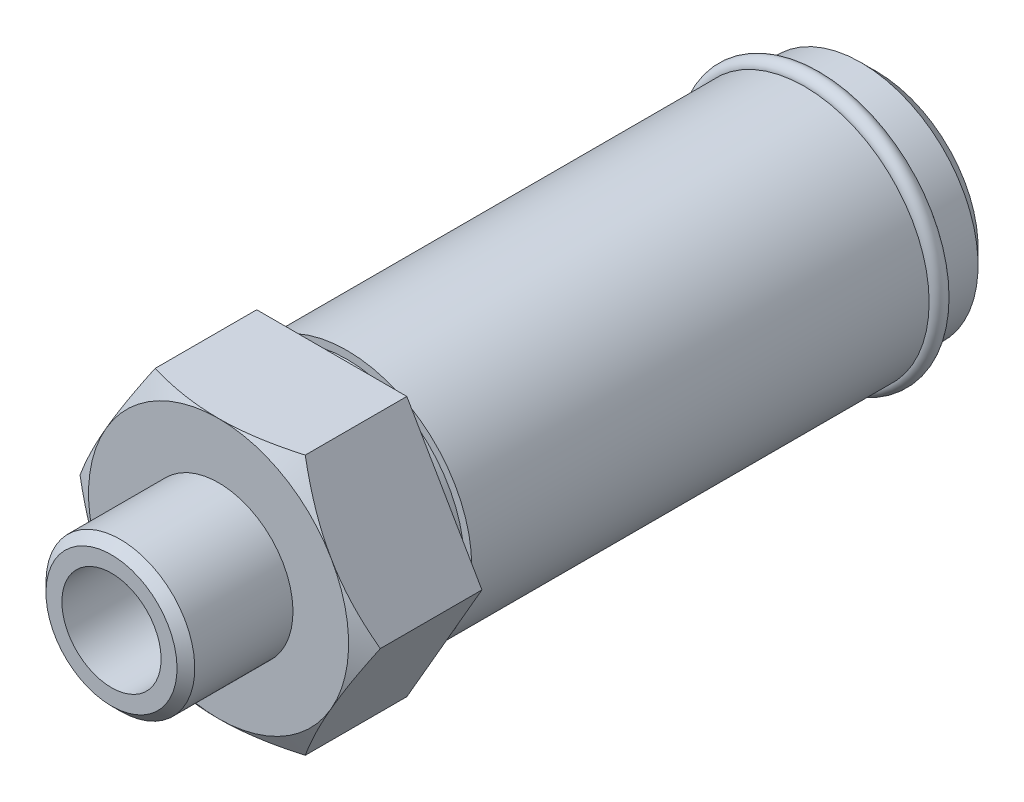
from build123d import *

# Parameters (mm, degrees)
CUT_EXTRUDE_START   = -7.4
SKETCH_2_R          = 17
CUT_EXTRUDE_1_DEPTH = 7.4


with BuildPart() as part:
    # 草图1 → 旋转1 (revolve)
    with BuildSketch(Plane(origin=(0, 0, 0), x_dir=(0, 0, -1), z_dir=(1, 0, 0)), mode=Mode.PRIVATE) as revolve_1_sk:
        with BuildLine():
            Line((-26.4, 0), (-26.4, 3.242666667))
            Line((-26.4, 3.242666667), (-46.4, 3.242666667))
            Line((-46.4, 3.242666667), (-46.4, 4.283))
            Line((-46.4, 4.283), (-45.819, 4.864))
            Line((-45.819, 4.864), (-39.4, 4.864))
            Line((-39.4, 4.864), (-39.4, 8.5))
            Line((-39.4, 8.5), (-34.492522712, 17))
            Line((-34.492522712, 17), (-32, 17))
            Line((-32, 17), (-32, 7.65))
            Line((-32, 7.65), (-31, 7.65))
            Line((-31, 7.65), (-31, 8.15))
            Line((-31, 8.15), (-1.099431524, 8.15))
            ThreePointArc((-1.099431524, 8.15), (-0.537496769, 8.674857863), (0, 8.125))
            Line((0, 8.125), (0, 7.65))
            Line((0, 7.65), (2.6, 7.65))
            Line((2.6, 7.65), (3.6, 6.65))
            Line((3.6, 6.65), (3.6, 4.864))
            Line((3.6, 4.864), (3.019, 4.283))
            Line((3.019, 4.283), (-2.9, 4.283))
            Line((-2.9, 4.283), (-2.9, 0))
            Line((-2.9, 0), (-26.4, 0))
        make_face()
    revolve(revolve_1_sk.sketch.rotate(Axis((0, 0, -3.6), (0, 0, 1)), 180), axis=Axis((0, 0, -3.6), (0, 0, 1)))

    # 草图2 → 切除-拉伸1 (cut)
    with BuildSketch(Plane.XY.offset(39.4).offset(CUT_EXTRUDE_START)):
        Circle(SKETCH_2_R)
        Polygon((-4.907477288, -8.5), (4.907477288, -8.5), (9.814954576, 0), (4.907477288, 8.5), (-4.907477288, 8.5), (-9.814954576, 0), align=None, mode=Mode.SUBTRACT)
    extrude(amount=CUT_EXTRUDE_1_DEPTH, mode=Mode.SUBTRACT)


solid = part.part
